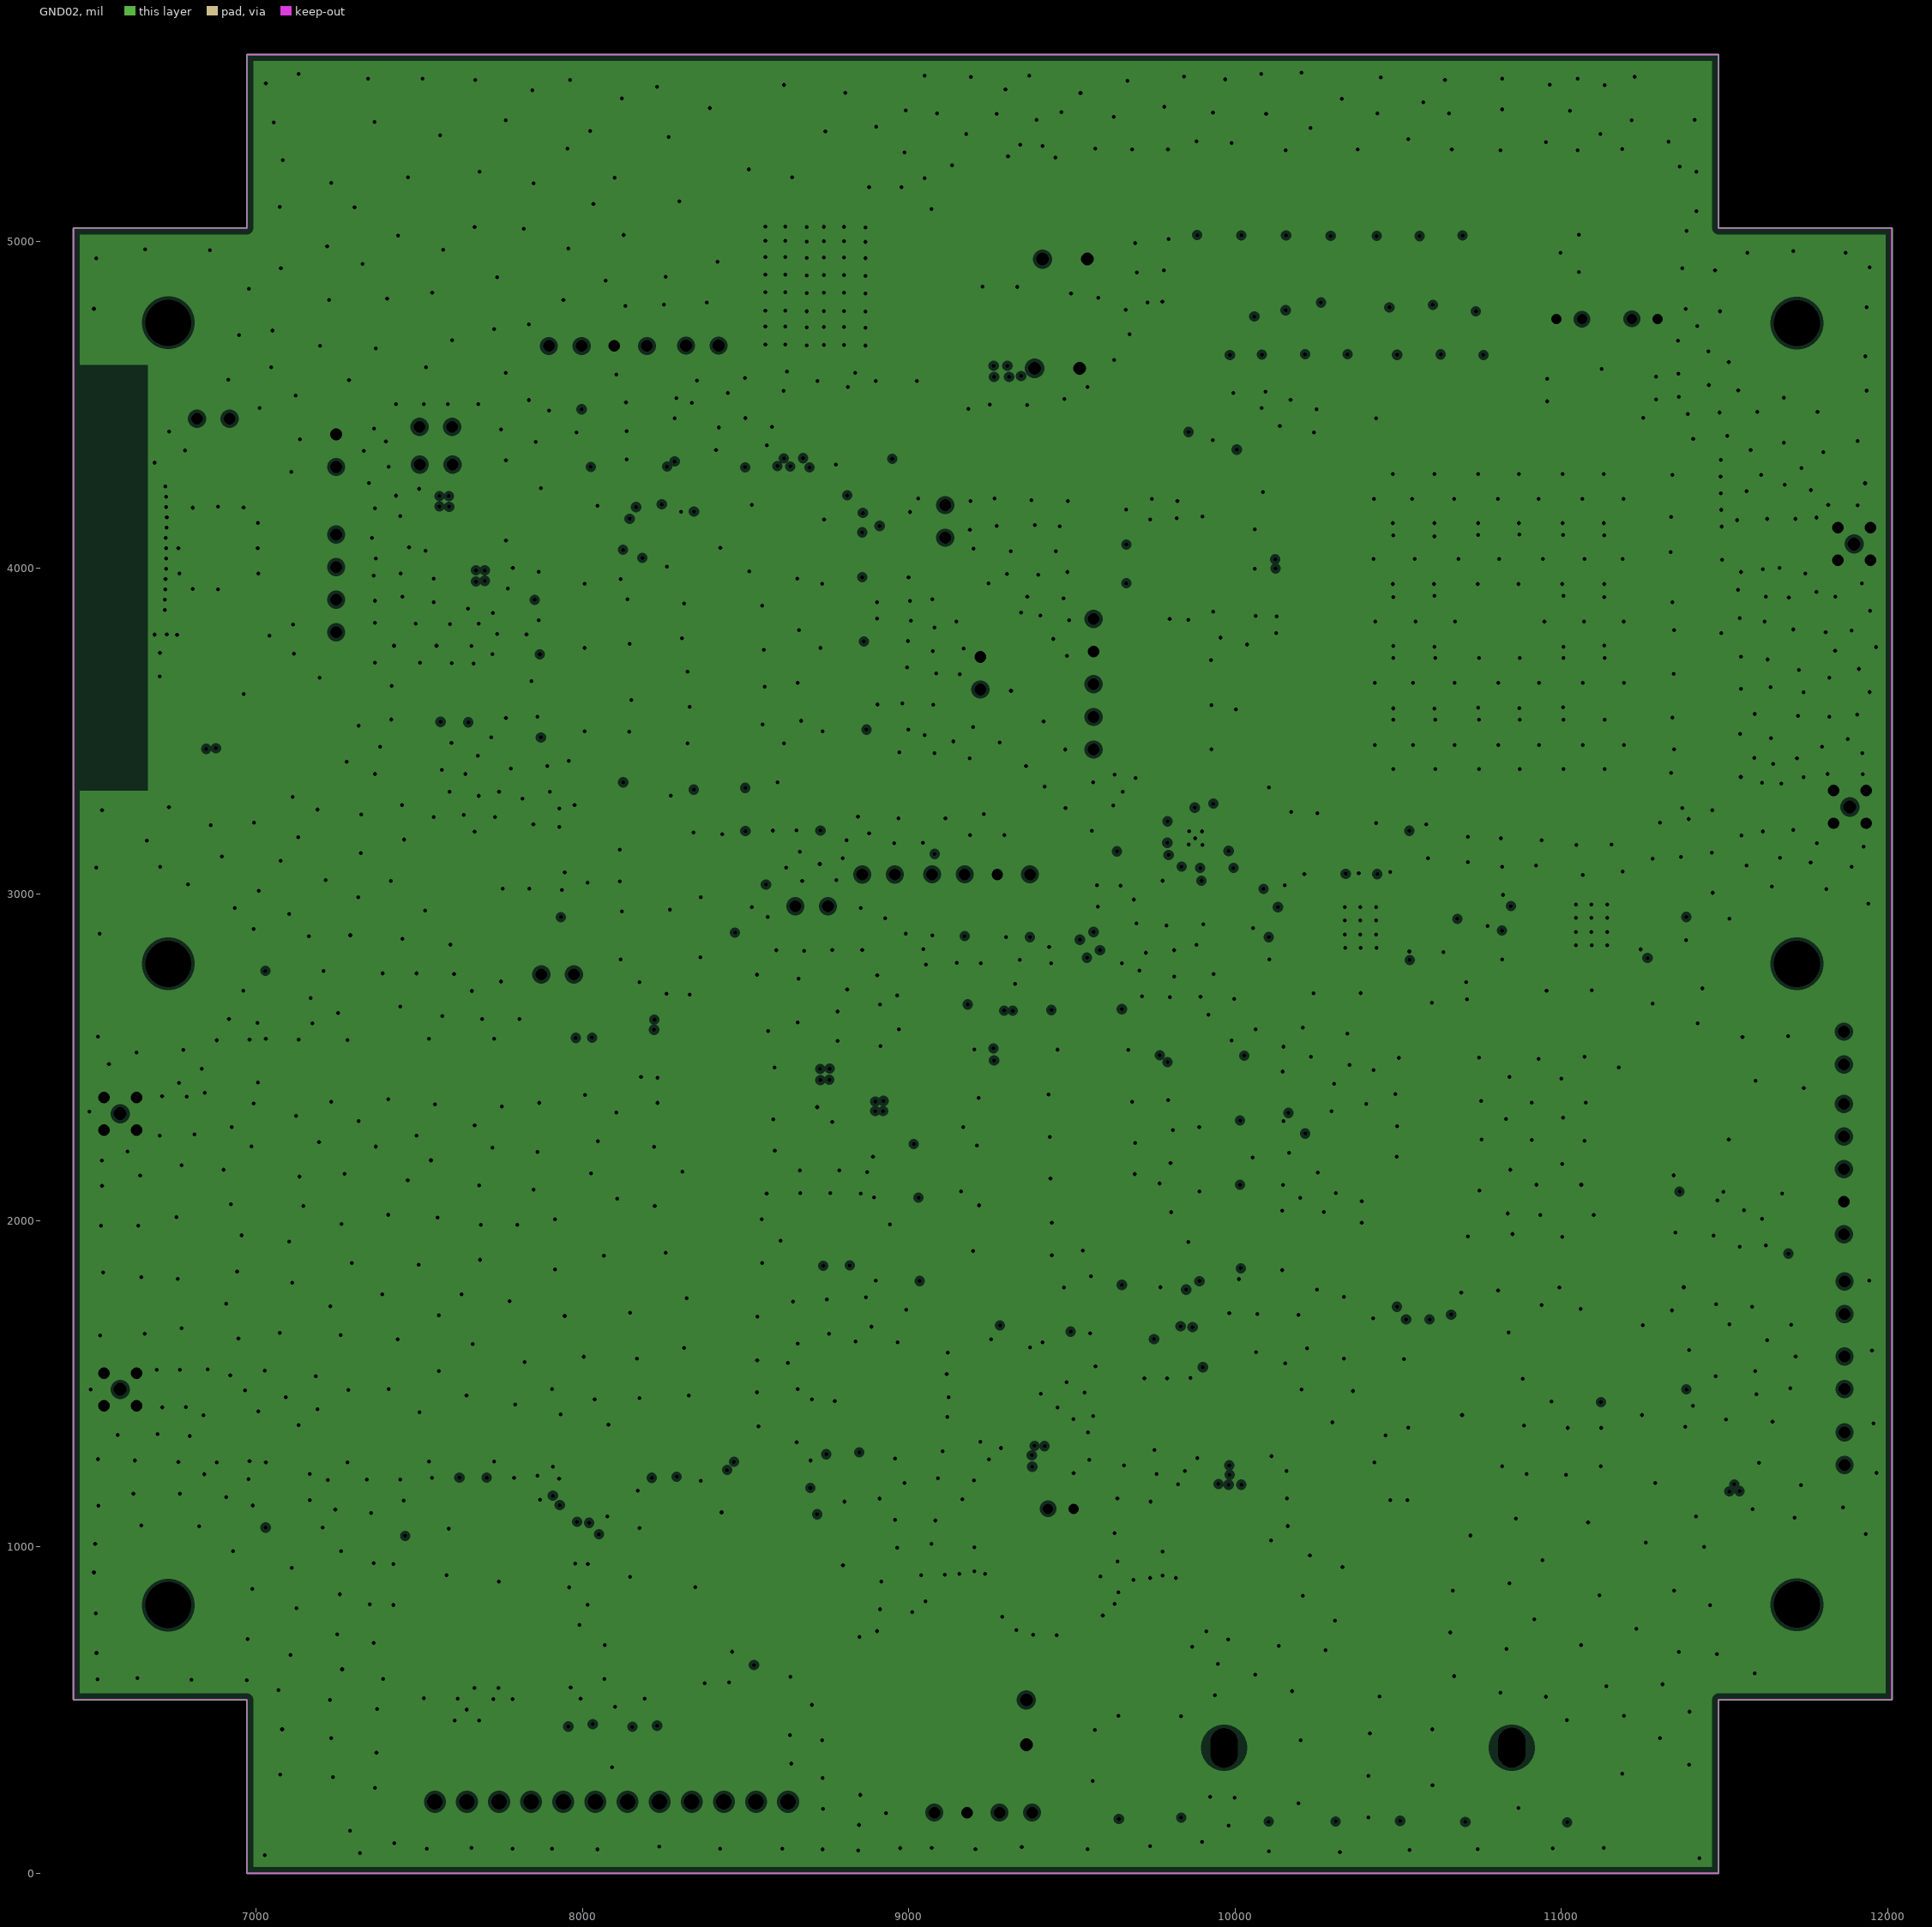
[diagram p0: GND02, clearances drawn from the general rule]
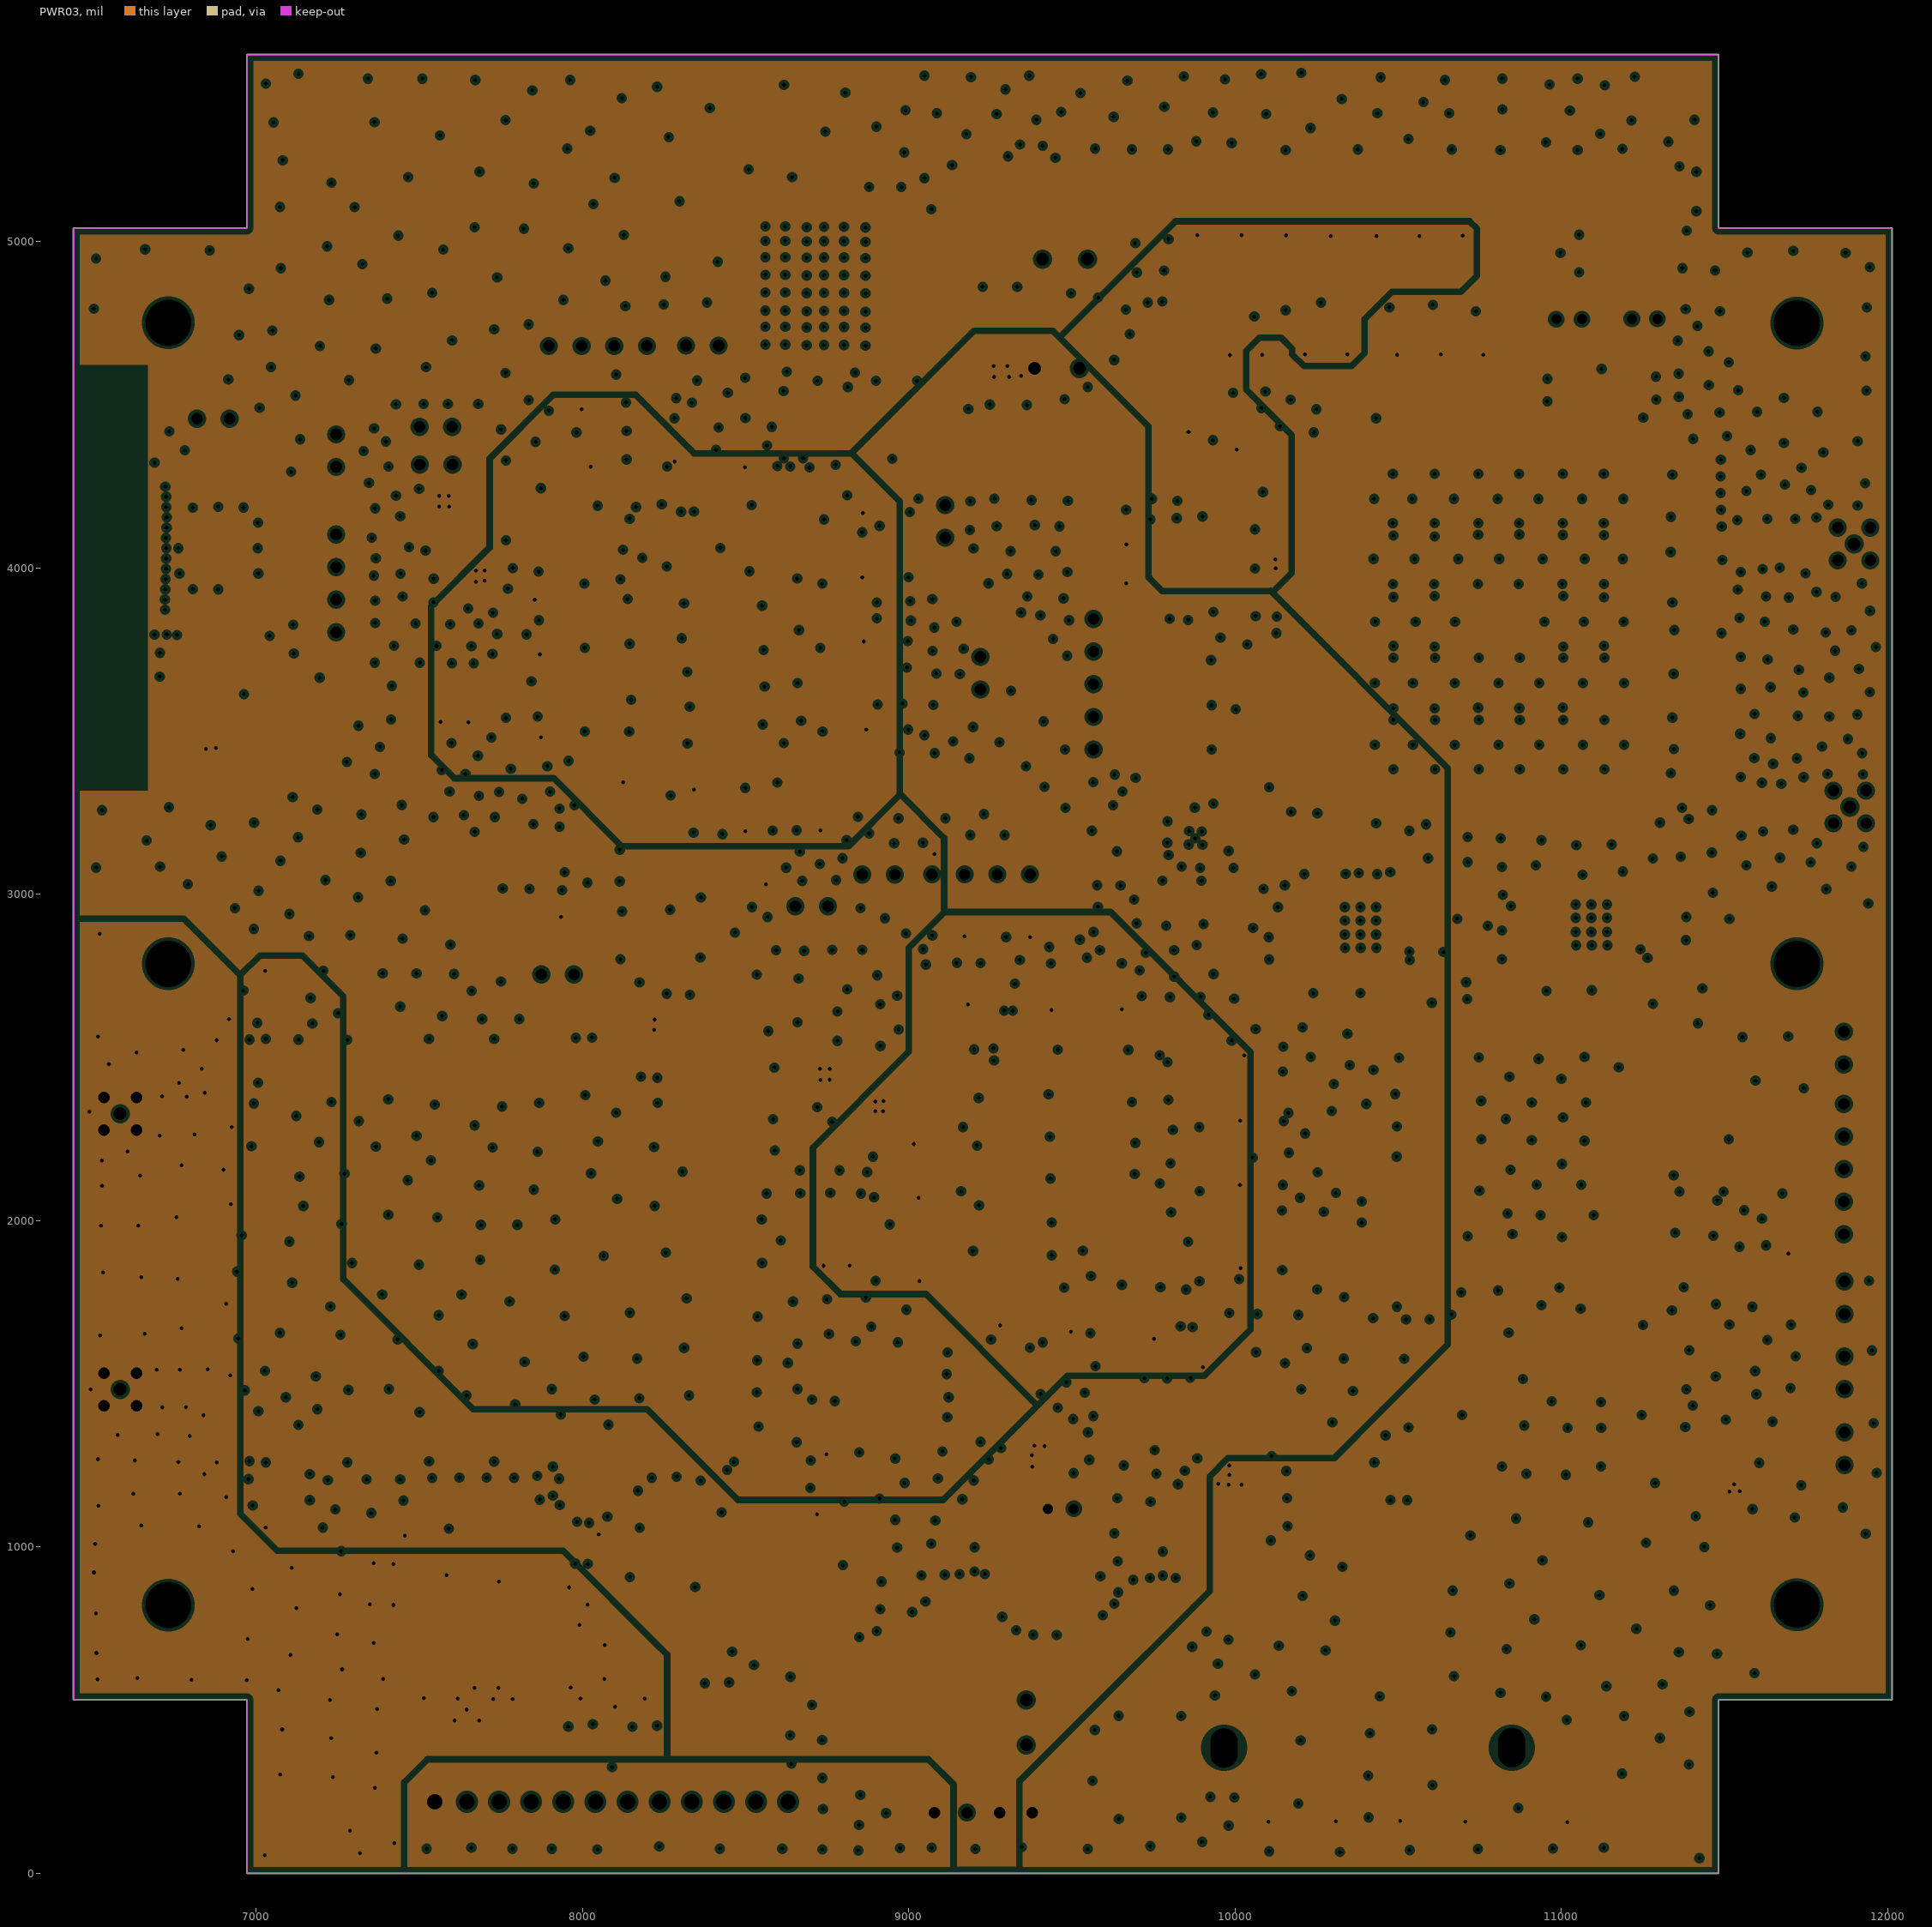
[diagram p1: PWR03, clearances drawn from the general rule]
# Altium PCB MISC86294.PcbDoc (part 2 of 8)
## Components (designator, comment, footprint, x,y, rotation, side; value= is the part's Value field where it differs from the comment) (continued)
R15 "10K" 0603 8499,3254 r270 top
R16 "10K" 0603 7808,3626 r270 top
R17 "120R@100MHz" 0603 8729,3254 r90 top
R18 "10K" 0603 8931.78,3695 r180 top
R19 "0R" 0603 7615,4141 r0 top
R20 "10K" 0603 7896.62,4543.46 r270 top
R21 "10K" 0603 7996.95,4545.83 r270 top
R22 "0R" R0603 11524,1220 r90 top
R23 "0R" R0603 11353,1477 r180 top
R24 "0R" R0603 10544,1647 r0 top
R25 "0R" R0603 11728,1893 r90 top
R26 "100K" 0603 9125,773 r270 top
R27 "75K 1%" 0603 9262,1057 r0 top
R28 "10K" 0603 9164,1085 r270 top
R29 "12V/2A" 1210 9097,570 r270 top
R30 "100K" 0603 9701,763 r270 top
R31 "100K" 0603 9843,1049 r0 top
R32 "1K" 0603 11018,217 r270 top
R33 "22.1K" 0603 9741,1076 r270 top
R34 "4.7K" R0603 10286.86,4921.68 r90 top
R35 "4.7K" R0603 9877.92,4921.68 r90 top
R36 "0R" R0603 11613.61,4081.3 r0 top
R37 "10K" R0603 10338.63,4678.78 r90 top
R38 "4.7K" R0603 10150.43,4921.68 r90 top
R39 "10K" R0603 9947.93,4676.78 r90 top
R40 "10K" R0603 10208.58,4678.78 r90 top
R41 "0R" R0603 10286.47,4750.82 r270 top
R42 "10K" R0603 10502.17,4750.82 r270 top
R43 "0R" R0603 10439.27,4750.82 r270 top
R44 "10K" R0603 10087.97,4750.82 r270 top
R45 "4.7K" R0603 10439.77,4993.72 r270 top
R46 "0R" R0603 11609.21,3274.94 r0 top
R47 "0R" R0603 10571.07,4750.82 r270 top
R48 "0R" R0603 10156.67,4750.82 r270 top
R49 "4.7K" R0603 10024.84,4993.72 r270 top
R50 "0R" R0603 10702.86,4750.82 r270 top
R51 "0R" R0603 10024.87,4750.82 r270 top
R52 "10K" R0603 10635.96,4750.82 r270 top
R53 "0R" R0603 9895.07,4749.82 r270 top
R54 "4.7K" R0603 10570.95,4993.72 r270 top
R55 "10K" R0603 10766.76,4750.82 r270 top
R56 "4.7K" R0603 10703.12,4993.72 r270 top
R57 "4.7K" R0603 10049.54,4369.59 r270 top
R58 "4.7K" R0603 9793.92,4391.44 r270 top
R59 "47K" R0603 9125.48,4602.83 r0 top
R60 "100K" R0603 9193.08,5136.79 r90 top
R61 "330R" R0603 9346.92,5268.52 r270 top
R62 "NM" R0603 10024.37,3601.94 r0 top
R63 "47K" R0603 9138.04,5208.85 r270 top
R64 "4.7K" R0603 10861.94,4750.82 r270 top
R65 "4.7K" R0603 9888.59,4078.35 r0 top
R66 "4.7K" R0603 9889.23,3959.35 r0 top
R67 "22R" R0603 10842.31,2938.79 r0 top
R68 "22R" R0603 10841.31,2876.32 r0 top
R69 "22R" R0603 11357.67,2925.13 r180 top
R70 "0R" R0603 6856.56,3483.52 r90 top
R71 "10K" R0603 6868.3,3677.56 r270 top
R72 "10K" R0603 6858.52,3747.44 r0 top
R73 "0R" R0603 7007.25,3749.4 r270 top
R74 "10K" R0603 7286.64,4203.56 r180 top
R75 "4.7Ω,±1%" 0603 7622.5,1150.2 r270 top
R76 "4.7Ω,±1%" 0603 8211.99,1145.2 r270 top
R77 "4.7Ω,±1%" 0603 7706.25,1150.2 r270 top
R78 "4.7Ω,±1%" 0603 8288.49,1145.2 r270 top
R79 "4.7Ω,±1%" 0603 7815.82,628.1 r90 top
R80 "22R" R0603 10128.31,2874.32 r0 top
R81 "4.7Ω,±1%" 0603 7890.7,628.1 r90 top
R82 "22R" R0603 10127.33,2934.87 r0 top
R83 "120R" R0603 8809.71,680.85 r180 top
R84 "NA" 0603 8494,3030 r180 top
R85 "10K" R0603 10525,3083 r0 top
R86 "10K" R0603 11122,2695 r90 top
R87 "10K" R0603 10431,2758 r270 top
R90 "22R" R0603 10649.05,2919.23 r180 top
R91 "NM" R0603 9751,3126 r90 top
R92 "NA" 0603 9834.55,239.87 r90 top
R93 "NA" 0603 9643.55,239.87 r90 top
R98 "NA" 0603 10705.49,217.71 r90 top
R200 "10R 1%" R0805 9358.87,1547.99 r180 top
R201 "10R 1%" R0805 8345.31,3116.89 r180 top
SW1 "TS-1101-B-W" SMD 7072.43,3444.04 r90 top
U1 "STM32F407ZET6" LQFP144-20x20mm 9525,2159 r0 top locked
U2 "STM32F103ZET6" LQFP144-20x20mm 8370.61,3824.32 r0 top
U3 "FSS-IMU614E-P1" FSS-IMU614E-P1 10950,2289 r180 top
U4 "SY8113B" TSOT-23-6_L2.9-W1.6-P0.95-LS2.8-BR 9201,915 r90 top
U5 "EC25/EC21_U17" EC20 10808,3836 r270 top
U6 "MIC29302WU" TO-263-5 8873.95,4862.15 r180 top
U7 "China Mobile eSIM" DFN-8_L6.0-W5.0-P1.27-BL-EP-A 11110.12,2904 r90 top
U8 "ESDA6V8V6-6" SOT-563 10770,2896 r90 top
U9 "SCC2130" SCC2130D 10972,1463.42 r270 top
U10 "ESP32-C3-MINI-1U" WIFIM-SMD_ESP32-C3-MINI-1 6883,4061 r90 top
U11 "SP3232EEN" SOP16-6_6 7710.45,893.36 r0 top
U12 "PESD15VL2BT" SOT-23 8064.3,548.15 r270 top
U13 "PESD15VL2BT" SOT-23 8260.45,548.4 r270 top
U14 "SP3232EEN" SOP16-6_6 8295.11,894.14 r0 top
U15 "PESD15VL2BT" SOT-23 7856.1,546.15 r270 top
U16 "SY8113B" TSOT-23-6_L2.9-W1.6-P0.95-LS2.8-BR 9778,901 r90 top
U17 "TJA1050T/CM,118" SOIC-8 8748.21,934.2 r180 top
U19 "China Telecom eSIM" DFN-8_L6.0-W5.0-P1.27-BL-EP-A 10400.92,2897.53 r90 top
U20 "FSA2567MPX" TQFN-16_L3.0-W3.0-P0.50-BL-EP1.7 9886.03,3173.04 r90 top
U21 "ESDA6V8V6-6" SOT-563 10046,2893 r90 top
Y1 "8MHZ 3.3V 20PPM" "XTAL 5.7X7.0-SM - duplicate" 9121.2,1464.37 r0 top
Y2 "8MHZ 3.3V 20PPM" "XTAL 5.7X7.0-SM - duplicate" 8112.63,3034.99 r0 top locked

## Footprints (in the part's own frame and the unit in brackets; to place one, negate y for a bottom-side part, rotate by r counter-clockwise, add the part's x,y. Pads: shape width x height; smd on the part's side, far side on the other; paste and mask are expansions set on the pad)
2.54mm_paizhen_5pin [mil]
  rect 59x59 hole 36: 1(0,200)
  round 59 hole 36: 2(0,100) 3(0,0) 4(0,-100) 5(0,-200)
  silkscreen extent -50,-250 50,250
0603 [mm]
  rect 0.8x0.9 smd: 1(-0.692,-0.003) 2(0.708,-0.003)
  silkscreen extent -1.4,-0.71 1.4,0.71
1210 [mm]
  rect 1.635x2.7 smd: 1(1.354,-0.12) 2(4.389,-0.12)
  silkscreen extent 0.31,-1.7 5.43,1.46
C0603 [mm]
  rect 0.8x0.9 smd: 1(-0.692,-0.003) 2(0.708,-0.003)
  silkscreen extent -1.4,-0.71 1.4,0.71
C0805 [mm]
  rect 1.41x1.35 smd: 1(-0.843,0) 2(1.217,0)
  silkscreen extent -1.78,-0.9 2.15,0.9
CAP-SMD_L3.5-W2.8 [mil]
  rect 63.29x93.54 smd: 1(71.01,0) 2(-71.01,0)
  silkscreen extent -72,-61 87,61
CAP-TH_BD5.0-P2.00-D0.8-FD [mm]
  round 1.3 hole 0.8: 1(-1,0) 2(1,0)
  silkscreen extent -2.5,-2.5 2.5,2.5
CAP-TH_BD8.0-P3.50-D1.0-FD [mm]
  round 1.6 hole 1: 1(-1.78,0) 2(1.72,0)
  silkscreen extent -4.03,-4.06 4.03,4.06
DFN-8_L6.0-W5.0-P1.27-BL-EP-A [mm]
  rect 0.45x1.1 smd: 1(-1.841,-2.417) 2(-0.571,-2.417) 3(0.699,-2.417) 4(1.968,-2.417) 5(1.968,3.183) 6(0.698,3.183) 7(-0.572,3.183) 8(-1.842,3.183)
  rect 4x3.4 smd: 9(0.063,0.384)
  silkscreen extent -2.6,-3.73 2.6,3.38
EC20 [mm]
  rect 0.8x1.625 smd: 1(-12.6,-16) 2(-11.3,-16) 3(-10,-16) 4(-8.7,-16) 5(-7.4,-16) 6(-6.1,-16) 7(-4.8,-16) 8(-0.4,-16) 9(0.9,-16) 10(2.2,-16) 11(3.5,-16) 12(4.8,-16) 13(6.1,-16) 14(7.4,-16) 15(8.7,-16) 16(10,-16) 17(11.3,-16) 18(12.6,-16) 37(12.6,16) 38(11.3,16) 39(10,16) 40(8.7,16) 41(7.4,16) 42(6.1,16) 43(4.8,16) 44(3.5,16) 45(2.2,16) 46(0.9,16) 47(-0.4,16) 48(-4.8,16) 49(-6.1,16) 50(-7.4,16) 51(-8.7,16) 52(-10,16) 53(-11.3,16) 54(-12.6,16) 141(-3,-16) 142(-1.7,-16) 143(-1.7,16) 144(-3,16)
  rect 1.625x0.8 smd: 19(14.5,-9.55) 20(14.5,-8.25) 21(14.5,-6.95) 22(14.5,-5.65) 23(14.5,-4.35) 24(14.5,-3.05) 25(14.5,-1.75) 26(14.5,-0.45) 27(14.5,0.85) 28(14.5,2.15) 29(14.5,3.45) 30(14.5,4.75) 31(14.5,6.05) 32(14.5,7.35) 33(14.5,8.65) 34(14.5,9.95) 35(14.5,11.25) 36(14.5,12.55) 55(-14.5,12.55) 56(-14.5,11.25) 57(-14.5,9.95) 58(-14.5,8.65) 59(-14.5,7.35) 60(-14.5,6.05) 61(-14.5,4.75) 62(-14.5,3.45) 63(-14.5,2.15) 64(-14.5,0.85) 65(-14.5,-0.45) 66(-14.5,-1.75) 67(-14.5,-3.05) 68(-14.5,-4.35) 69(-14.5,-5.65) 70(-14.5,-6.95) 71(-14.5,-8.25) 72(-14.5,-9.55) 113(-14.5,-10.85) 114(-14.5,-12.15) 115(14.5,-10.85) 116(14.5,-12.15)
  rect 3x2 smd: 85(-9.6,8.2) 86(-4.8,8.2) 87(0,8.2) 88(4.8,8.2) 89(9.6,8.2) 90(-9.6,5) 91(-4.8,5) 92(0,5) 93(4.8,5) 94(9.6,5) 95(-9.6,1.6) 96(-4.8,1.6) 97(4.8,1.6) 98(9.6,1.6) 99(-9.6,-1.6) 100(-4.8,-1.6) 101(4.8,-1.6) 102(9.6,-1.6) 103(-9.6,-5) 104(-4.8,-5) 105(0,-5) 106(4.8,-5) 107(9.6,-5) 108(-9.6,-8.2) 109(-4.8,-8.2) 110(0,-8.2) 111(4.8,-8.2) 112(9.6,-8.2)
  rect 1.1x1.1 smd: 117(-11,-11) 118(-9,-11) 119(-7,-11) 120(-5,-11) 121(-3,-11) 122(-1,-11) 123(1,-11) 124(3,-11) 125(5,-11) 126(7,-11) 127(9,-11) 128(11,-11) 129(-11,-13) 130(-9,-13) 131(-7,-13) 132(-5,-13) 133(-3,-13) 134(-1,-13) 135(1,-13) 136(3,-13) 137(5,-13) 138(7,-13) 139(9,-13) 140(11,-13)
  silkscreen extent -15.1,-16.6 14.7,16.1
EMT3 [mm]
  rect 0.65x0.46 smd: 1(0.525,0.5) 2(0.525,-0.5) 3(-0.525,0)
  silkscreen extent -0.37,-0.8 0.42,0.8
FSS-IMU614E-P1 [mm]
  rect 2x0.85 smd: 1(-8.5,5.08) 2(-8.5,3.81) 3(-8.5,2.54) 4(-8.5,1.27) 5(-8.5,0) 6(-8.5,-1.27) 7(-8.5,-2.54) 8(-8.5,-3.81) 9(-8.5,-5.08) 10(8.5,-5.08) 11(8.5,-3.81) 12(8.5,-2.54) 13(8.5,-1.27) 14(8.5,0) 15(8.5,1.27) 16(8.5,2.54) 17(8.5,3.81) 18(8.5,5.08)
  silkscreen extent -10.92,-7.5 8.5,7.5
HDR1X4 [mm] "Connector; Header; 4 Position"
  rect 1.5x1.5 hole 0.9: 1(0,0)
  round 1.5 hole 0.9: 2(2.54,0) 3(5.08,0) 4(7.62,0)
  silkscreen extent -1.27,-1.27 8.89,1.27
HDR_1X2_254 [mil]
  rect 59x59 hole 36: 1(-50,0)
  round 59 hole 36: 2(50,0)
  silkscreen extent -100,-50 100,50
HDR_1X4_254 [mil]
  rect 59x59 hole 36: 1(-150,0)
  round 59 hole 36: 2(-50,0) 3(50,0) 4(150,0)
  silkscreen extent -200,-50 200,50
IND-SMD_L4.0-W4.0 [mm]
  rect 1.6x3.5 smd: 1(-1.6,0) 2(1.6,0)
  silkscreen extent -2.08,-2.1 2.08,2.1
LED0805 [mil]
  rect 51.2x55.1 smd: 1(-45.9,-0.55) 2(36.8,-0.55)
  silkscreen extent -83,-41 83,41
LED_0805 [mil]
  rect 51.2x55.1 smd: 1(-45.9,-0.55) 2(36.8,-0.55)
  silkscreen extent -83,-41 83,41
LQFP144-20x20mm [mm]
  oval 0.28x2 smd: 1(-8.75,-10.8) 2(-8.25,-10.8) 3(-7.75,-10.8) 4(-7.25,-10.8) 5(-6.75,-10.8) 6(-6.25,-10.8) 7(-5.75,-10.8) 8(-5.25,-10.8) 9(-4.75,-10.8) 10(-4.25,-10.8) 11(-3.75,-10.8) 12(-3.25,-10.8) 13(-2.75,-10.8) 14(-2.25,-10.8) 15(-1.75,-10.8) 16(-1.25,-10.8) 17(-0.75,-10.8) 18(-0.25,-10.8) 19(0.25,-10.8) 20(0.75,-10.8) 21(1.25,-10.8) 22(1.75,-10.8) 23(2.25,-10.8) 24(2.75,-10.8) 25(3.25,-10.8) 26(3.75,-10.8) 27(4.25,-10.8) 28(4.75,-10.8) 29(5.25,-10.8) 30(5.75,-10.8) 31(6.25,-10.8) 32(6.75,-10.8) 33(7.25,-10.8) 34(7.75,-10.8) 35(8.25,-10.8) 36(8.75,-10.8) 73(8.75,10.8) 74(8.25,10.8) 75(7.75,10.8) 76(7.25,10.8) 77(6.75,10.8) 78(6.25,10.8) 79(5.75,10.8) 80(5.25,10.8) 81(4.75,10.8) 82(4.25,10.8) 83(3.75,10.8) 84(3.25,10.8) 85(2.75,10.8) 86(2.25,10.8) 87(1.75,10.8) 88(1.25,10.8) 89(0.75,10.8) 90(0.25,10.8) 91(-0.25,10.8) 92(-0.75,10.8) 93(-1.25,10.8) 94(-1.75,10.8) 95(-2.25,10.8) 96(-2.75,10.8) 97(-3.25,10.8) 98(-3.75,10.8) 99(-4.25,10.8) 100(-4.75,10.8) 101(-5.25,10.8) 102(-5.75,10.8) 103(-6.25,10.8) 104(-6.75,10.8) 105(-7.25,10.8) 106(-7.75,10.8) 107(-8.25,10.8) 108(-8.75,10.8)
  oval 2x0.28 smd: 37(10.8,-8.75) 38(10.8,-8.25) 39(10.8,-7.75) 40(10.8,-7.25) 41(10.8,-6.75) 42(10.8,-6.25) 43(10.8,-5.75) 44(10.8,-5.25) 45(10.8,-4.75) 46(10.8,-4.25) 47(10.8,-3.75) 48(10.8,-3.25) 49(10.8,-2.75) 50(10.8,-2.25) 51(10.8,-1.75) 52(10.8,-1.25) 53(10.8,-0.75) 54(10.8,-0.25) 55(10.8,0.25) 56(10.8,0.75) 57(10.8,1.25) 58(10.8,1.75) 59(10.8,2.25) 60(10.8,2.75) 61(10.8,3.25) 62(10.8,3.75) 63(10.8,4.25) 64(10.8,4.75) 65(10.8,5.25) 66(10.8,5.75) 67(10.8,6.25) 68(10.8,6.75) 69(10.8,7.25) 70(10.8,7.75) 71(10.8,8.25) 72(10.8,8.75) 109(-10.8,8.75) 110(-10.8,8.25) 111(-10.8,7.75) 112(-10.8,7.25) 113(-10.8,6.75) 114(-10.8,6.25) 115(-10.8,5.75) 116(-10.8,5.25) 117(-10.8,4.75) 118(-10.8,4.25) 119(-10.8,3.75) 120(-10.8,3.25) 121(-10.8,2.75) 122(-10.8,2.25) 123(-10.8,1.75) 124(-10.8,1.25) 125(-10.8,0.75) 126(-10.8,0.25) 127(-10.8,-0.25) 128(-10.8,-0.75) 129(-10.8,-1.25) 130(-10.8,-1.75) 131(-10.8,-2.25) 132(-10.8,-2.75) 133(-10.8,-3.25) 134(-10.8,-3.75) 135(-10.8,-4.25) 136(-10.8,-4.75) 137(-10.8,-5.25) 138(-10.8,-5.75) 139(-10.8,-6.25) 140(-10.8,-6.75) 141(-10.8,-7.25) 142(-10.8,-7.75) 143(-10.8,-8.25) 144(-10.8,-8.75)
  silkscreen extent -10.41,-11.25 10.08,10.08
MMCX-KE [mm]
  round 1.524 hole 1: 1(0,0)
  round 1.4 hole 0.9: 2(-1.27,1.27) 3(-1.27,-1.27) 4(1.27,-1.27) 5(1.27,1.27)
  silkscreen extent -1.78,-1.78 1.78,1.78
R0603 [mil]
  rect 31.75x34.02 smd: 1(6.36,-5.87) 2(65.67,-5.87)
  silkscreen extent -19,-32 91,20
R0805 [mil]
  rect 44.59x54.21 smd: 1(-38.04,0) 2(38.04,0)
  silkscreen extent -69,-36 69,36
RB5*7 [mm]
  round 1.3 hole 0.8: 1(-1,0) 2(1,0)
  silkscreen extent -2.5,-2.5 2.5,2.5
RB8*11_5 [mm]
  round 1.6 hole 1: 1(-1.769,-0.001) 2(1.731,-0.001)
  silkscreen extent -3.98,-4 4.02,4